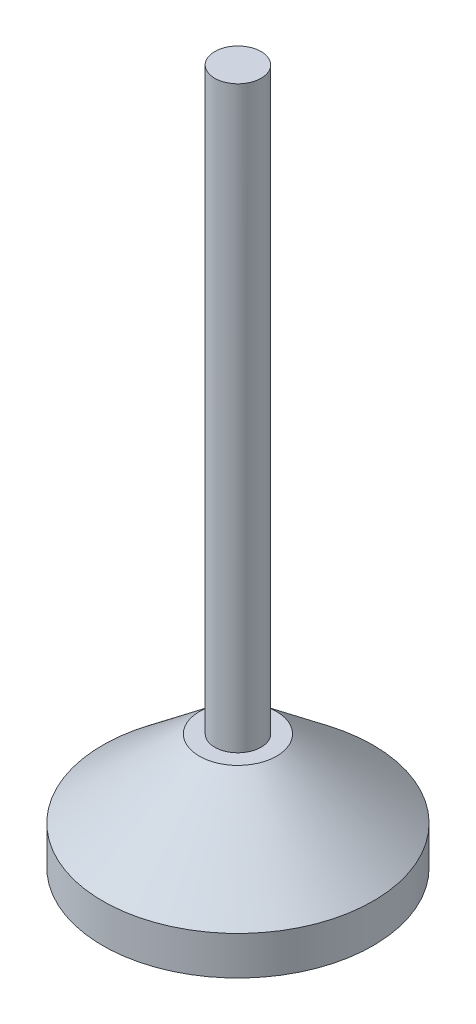
from build123d import *

# Parameters (mm, degrees)
SKETCH_1_R      = 6
EXTRUDE_1_DEPTH = 150
SKETCH_2_R      = 35
EXTRUDE_2_DEPTH = 30
CHAMFER_1_SIZE  = 25
CHAMFER_1_SIZE2 = 20


with BuildPart() as part:
    # 草图1 → 凸台-拉伸1 (new body)
    with BuildSketch(Plane(origin=(0, 0, 0), x_dir=(1, 0, 0), z_dir=(0, 1, 0))):
        with Locations(Location((0, 0, 0), (0, 0, 270))):
            Circle(SKETCH_1_R)
    extrude(amount=EXTRUDE_1_DEPTH)

    # 草图2 → 凸台-拉伸2 (add)
    with BuildSketch(Plane.XZ):
        with Locations(Location((0, 0, 0), (0, 0, 270))):
            Circle(SKETCH_2_R)
    extrude(amount=EXTRUDE_2_DEPTH)

    # 倒角1
    chamfer_1_edges = [part.edges().sort_by_distance(p)[0] for p in [
        (0, 0, 35),
    ]]
    chamfer_1_side = [part.faces().sort_by_distance(p)[0] for p in [
        (0, 0, 34.010050506),
    ]]
    chamfer(chamfer_1_edges, length=CHAMFER_1_SIZE, length2=CHAMFER_1_SIZE2, reference=chamfer_1_side[0])


solid = part.part
